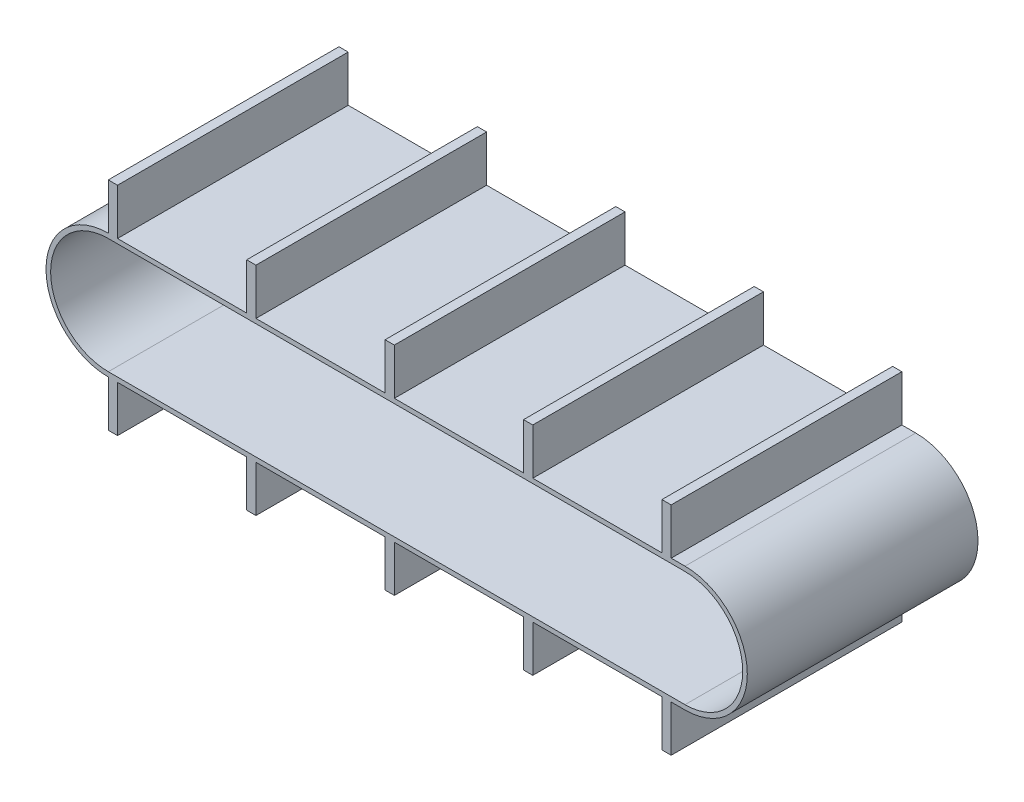
from build123d import *

# Parameters (mm, degrees)
EXTRUDE_1_DEPTH        = 100
SKETCH_2_W             = 4
SKETCH_2_H             = 20
EXTRUDE_2_DEPTH        = 100
PATTERN_LINEAR_1_COUNT = 5
PATTERN_LINEAR_1_PITCH = 60
SKETCH_3_W             = 4
SKETCH_3_H             = 20
EXTRUDE_3_DEPTH        = 100
PATTERN_LINEAR_2_COUNT = 5
PATTERN_LINEAR_2_PITCH = 60


with BuildPart() as part:
    # 草图1 → 凸台-拉伸1 (new body)
    with BuildSketch(Plane.XY):
        with BuildLine():
            Line((0, 27), (250, 27))
            ThreePointArc((250, 27), (277, 0), (250, -27))
            Line((250, -27), (0, -27))
            ThreePointArc((0, -27), (-27, 0), (0, 27))
        make_face()
        with BuildLine():
            Line((0, 25), (250, 25))
            ThreePointArc((250, 25), (275, 0), (250, -25))
            Line((250, -25), (0, -25))
            ThreePointArc((0, -25), (-25, 0), (0, 25))
        make_face(mode=Mode.SUBTRACT)
    extrude(amount=EXTRUDE_1_DEPTH)

    # 草图2 → 凸台-拉伸2 (add)
    with BuildSketch(Plane.XY.offset(100)):
        with Locations((2, 37)):
            Rectangle(SKETCH_2_W, SKETCH_2_H)
    extrude_2 = extrude(amount=-EXTRUDE_2_DEPTH)

    # 阵列(线性)1: 凸台-拉伸2 ×5
    with Locations(*[(i * PATTERN_LINEAR_1_PITCH, 0, 0) for i in range(1, PATTERN_LINEAR_1_COUNT)]):
        add(extrude_2)

    # 草图3 → 凸台-拉伸3 (add)
    with BuildSketch(Plane.XY.offset(100)):
        with Locations((2, -37)):
            Rectangle(SKETCH_3_W, SKETCH_3_H)
    extrude_3 = extrude(amount=-EXTRUDE_3_DEPTH)

    # 阵列(线性)2: 凸台-拉伸3 ×5
    with Locations(*[(i * PATTERN_LINEAR_2_PITCH, 0, 0) for i in range(1, PATTERN_LINEAR_2_COUNT)]):
        add(extrude_3)


solid = part.part
